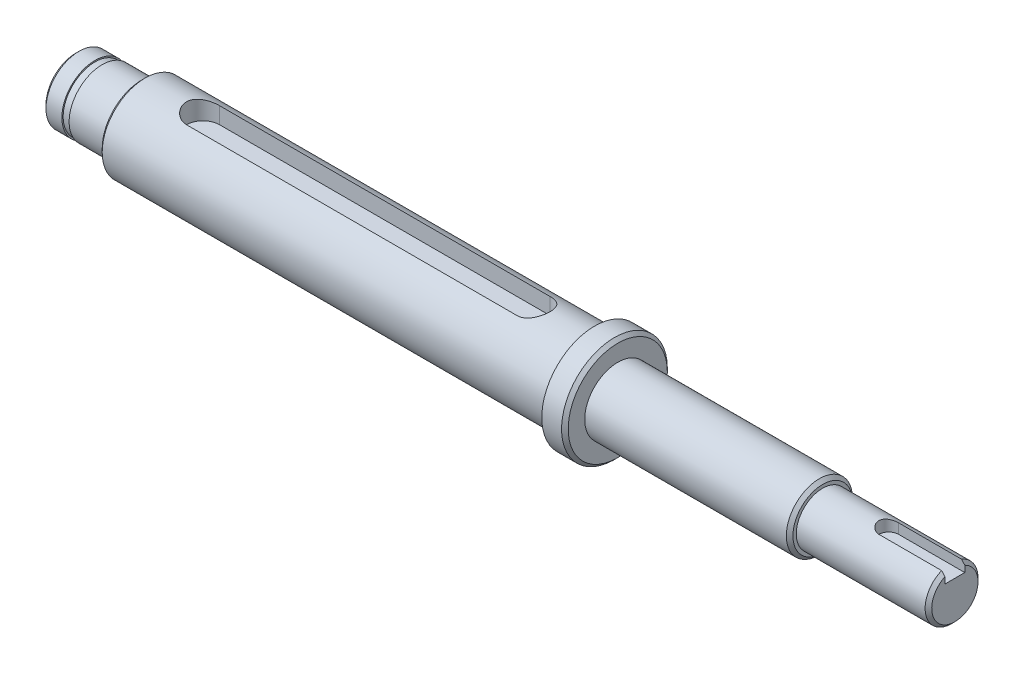
SolidWorks part; units mm, degrees
material "45#"
ref_plane "前基準面" through (0, 0, 0) normal (0, 0, 1) x (1, 0, 0)
ref_plane "上基準面" through (0, 0, 0) normal (0, 1, 0) x (1, 0, 0)
ref_plane "右基準面" through (0, 0, 0) normal (1, 0, 0) x (0, 0, -1)
sketch "草图1" plane through (0, 0, 0) normal (0, 0, 1) x (1, 0, 0)
  line L0 (0, 0) -> (-133.0184, 0) construction
  line L1 (0, 0) -> (0, 12.0185) construction
  line L4 (-133, 5) -> (-130.1, 5)
  line L5 (0, 4) -> (0, 0)
  line L9 (-133, 5) -> (-133, 0)
  line L10 (-133, 0) -> (0, 0)
  line L11 (-129, 5) -> (-129, 4.8)
  line L12 (-129, 4.8) -> (-130.1, 4.8)
  line L13 (-130.1, 4.8) -> (-130.1, 5)
  line L14 (-129, 5) -> (-123, 5)
  line L19 (0, 4) -> (-20, 4)
  line L20 (-20, 4) -> (-20, 5)
  line L21 (-51, 5) -> (-51, 8)
  line L22 (-54.5, 6.5) -> (-123, 6.5)
  line L23 (-123, 6.5) -> (-123, 5)
  line L24 (-51, 5) -> (-20, 5)
  line L25 (-54.5, 6.5) -> (-54.5, 8)
  line L26 (-54.5, 8) -> (-51, 8)
  dimension "D13" = 72
  dimension "D2" = 13
  dimension "D3" = 9.6
  dimension "D4" = 1.1
  dimension "D5" = 10
  dimension "D6" = 3.5
  dimension "D7" = 8
  dimension "D8" = 20
  dimension "D9" = 31
  dimension "D10" = 6
  dimension "D11" = 10
  dimension "D12" = 2.9
  dimension "D14" = 16
revolve "旋转1" add sketch "草图1" angle 360 about L0
sketch "草图2" plane through (0, 0, 0) normal (0, 1, 0) x (1, 0, 0)
  line L0 (-10, 0) -> (0, 0) construction
  line L1 (-10, 1.5) -> (0, 1.5)
  line L2 (-10, -1.5) -> (0, -1.5)
  arc A0 (-10, 1.5) -> (-10, -1.5) centre (-10, 0) ccw
  arc A1 (0, -1.5) -> (0, 1.5) centre (0, 0) ccw
  point P2 (-5, 0)
  dimension "D2" = 1.5
  dimension "D1" = 10
extrude "切除-拉伸1" cut sketch "草图2" against normal blind 1.8 from offset 4
chamfer "倒角1" distance 0.5 angle 45 5 edges at (-133, 0, -5) (0, -4, 0) (-123, 0, -6.5) (-20, 0, -5) (-51, 0, -8)
ref_plane "基准面1" through (0, 6.5, 0) normal (0, 1, 0) x (1, 0, 0)
sketch "草图4" plane through (0, 6.5, 0) normal (0, 1, 0) x (1, 0, 0)
  line L0 (-113.75, 0) -> (-63.75, 0) construction
  line L1 (-113.75, 2.5) -> (-63.75, 2.5)
  line L2 (-113.75, -2.5) -> (-63.75, -2.5)
  line L3 (-54.5, 0) -> (-123, 0) construction
  line L4 (-54.5, 6.5) -> (-54.5, -6.5) construction
  line L5 (-123, 5) -> (-123, -5) construction
  arc A0 (-113.75, 2.5) -> (-113.75, -2.5) centre (-113.75, 0) ccw
  arc A1 (-63.75, -2.5) -> (-63.75, 2.5) centre (-63.75, 0) ccw
  point P2 (-88.75, 0)
  dimension "D1" = 5
  dimension "D2" = 50
extrude "切除-拉伸3" cut sketch "草图4" against normal blind 3
